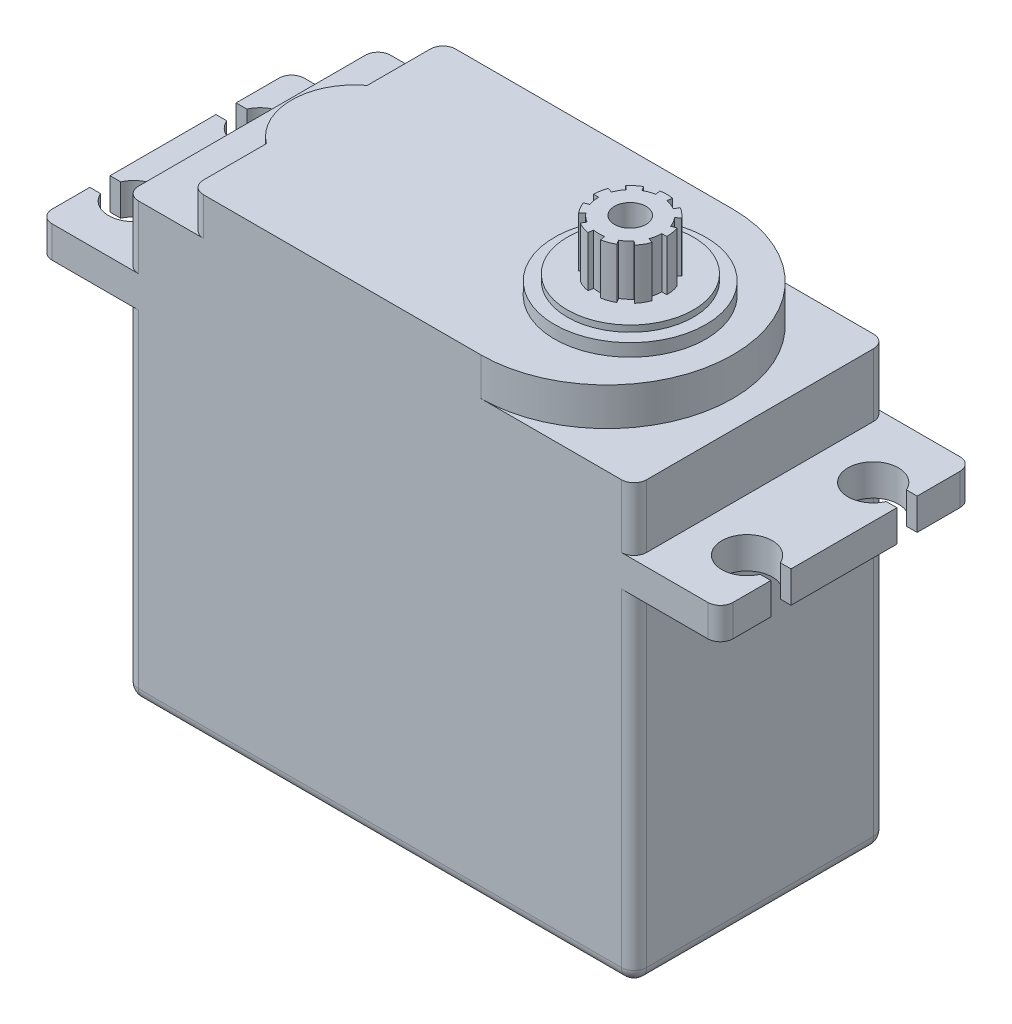
from build123d import *

# Parameters (mm, degrees)
EXTRUDE_1_DEPTH        = 20
FILLET_1_R             = 1
CUT_EXTRUDE_1_DEPTH    = 20
SKETCH_3_W             = 51.867663345
SKETCH_3_H             = 35.261757523
CUT_EXTRUDE_2_DEPTH    = 3
SKETCH_4_R             = 6
EXTRUDE_2_DEPTH        = 1
SKETCH_5_R             = 5
EXTRUDE_3_DEPTH        = 0.5
SKETCH_6_R             = 1
EXTRUDE_4_DEPTH        = 4
HOLE_WIZARD_M3_1_D     = 2.5
HOLE_WIZARD_M3_1_DEPTH = 7.5
HOLE_WIZARD_M3_1_TIP   = 0.751075774


with BuildPart() as part:
    # 草图1 → 凸台-拉伸1 (new body)
    with BuildSketch(Plane.XY):
        Polygon((20.15, 8), (27, 8), (27, 10.5), (20.15, 10.5), (20.15, 18.5), (-20.15, 18.5), (-20.15, 10.5), (-27, 10.5), (-27, 8), (-20.15, 8), (-20.15, -19), (20.15, -19), align=None)
    extrude(amount=EXTRUDE_1_DEPTH)

    # 圆角1
    fillet_1_edges = [part.edges().sort_by_distance(p)[0] for p in [
        (-27, 9.25, 20),
        (20.15, 14.5, 0),
        (27, 9.25, 0),
        (20.15, -5.5, 0),
        (0, -19, 0),
        (-20.15, -5.5, 0),
        (-27, 9.25, 0),
        (-20.15, 14.5, 0),
        (-20.15, -5.5, 20),
        (0, -19, 20),
        (-20.15, 18.5, 10),
        (20.15, 18.5, 10),
        (20.15, -19, 10),
        (-20.15, -19, 10),
        (20.15, -5.5, 20),
        (27, 9.25, 20),
        (20.15, 14.5, 20),
        (-20.15, 14.5, 20),
    ]]
    fillet(fillet_1_edges, radius=FILLET_1_R)

    # 草图2 → 切除-拉伸1 (cut)
    with BuildSketch(Plane(origin=(0, 10.5, 0), x_dir=(1, 0, 0), z_dir=(0, 1, 0))):
        with BuildLine():
            Line((-26.148030278, -4.4), (-29.222738853, -4.4))
            Line((-29.222738853, -4.4), (-29.222738853, -6))
            Line((-29.222738853, -6), (-26.148030278, -6))
            ThreePointArc((-26.148030278, -6), (-22.315, -5.2), (-26.148030278, -4.4))
        make_face()
        with BuildLine():
            Line((-26.148030278, -14.4), (-29.222738853, -14.4))
            Line((-29.222738853, -14.4), (-29.222738853, -16))
            Line((-29.222738853, -16), (-26.148030278, -16))
            ThreePointArc((-26.148030278, -16), (-22.315, -15.2), (-26.148030278, -14.4))
        make_face()
        with BuildLine():
            Line((26.148030278, -16), (29.222738853, -16))
            Line((29.222738853, -16), (29.222738853, -14.4))
            Line((29.222738853, -14.4), (26.148030278, -14.4))
            ThreePointArc((26.148030278, -14.4), (22.315, -15.2), (26.148030278, -16))
        make_face()
        with BuildLine():
            Line((29.222738853, -4.4), (29.222738853, -6))
            Line((29.222738853, -6), (26.148030278, -6))
            ThreePointArc((26.148030278, -6), (22.315, -5.2), (26.148030278, -4.4))
            Line((26.148030278, -4.4), (29.222738853, -4.4))
        make_face()
    extrude(amount=-CUT_EXTRUDE_1_DEPTH, mode=Mode.SUBTRACT)

    # 草图3 → 切除-拉伸2 (cut)
    with BuildSketch(Plane(origin=(0, 18.5, 0), x_dir=(1, 0, 0), z_dir=(0, 1, 0))):
        with Locations((-0.933831673, -10.85793672)):
            Rectangle(SKETCH_3_W, SKETCH_3_H)
        with BuildLine():
            Line((-14, 0), (8, 0))
            ThreePointArc((8, 0), (18, -10), (8, -20))
            Line((8, -20), (-14, -20))
            ThreePointArc((-14, -20), (-14.707106781, -19.707106781), (-15, -19))
            Line((-15, -19), (-15, -14))
            ThreePointArc((-15, -14), (-17, -10), (-15, -6))
            Line((-15, -6), (-15, -1))
            ThreePointArc((-15, -1), (-14.707106781, -0.292893219), (-14, 0))
        make_face(mode=Mode.SUBTRACT)
    extrude(amount=-CUT_EXTRUDE_2_DEPTH, mode=Mode.SUBTRACT)

    # 草图4 → 凸台-拉伸2 (add)
    with BuildSketch(Plane(origin=(0, 18.5, 0), x_dir=(1, 0, 0), z_dir=(0, 1, 0))):
        with Locations((9.85, -10)):
            Circle(SKETCH_4_R)
    extrude(amount=EXTRUDE_2_DEPTH)

    # 草图5 → 凸台-拉伸3 (add)
    with BuildSketch(Plane(origin=(0, 19.5, 0), x_dir=(1, 0, 0), z_dir=(0, 1, 0))):
        with Locations(Location((9.851314919, -9.987632383, 0), (0, 0, 270))):
            Circle(SKETCH_5_R)
    extrude(amount=EXTRUDE_3_DEPTH)

    # 草图6 → 凸台-拉伸4 (add)
    with BuildSketch(Plane(origin=(0, 20, 0), x_dir=(1, 0, 0), z_dir=(0, 1, 0))):
        with BuildLine():
            Line((10.284120444, -7.537980617), (10.353579715, -7.144057516))
            ThreePointArc((10.353579715, -7.144057516), (9.85, -7.1), (9.346420285, -7.144057516))
            Line((9.346420285, -7.144057516), (9.415879556, -7.537980617))
            ThreePointArc((9.415879556, -7.537980617), (8.994949642, -7.650768448), (8.6, -7.834936491))
            Line((8.6, -7.834936491), (8.4, -7.488526329))
            ThreePointArc((8.4, -7.488526329), (7.985915932, -7.778471115), (7.628471115, -8.135915932))
            Line((7.628471115, -8.135915932), (7.934888892, -8.393030976))
            ThreePointArc((7.934888892, -8.393030976), (7.684936491, -8.75), (7.500768448, -9.144949642))
            Line((7.500768448, -9.144949642), (7.1248914, -9.008141584))
            ThreePointArc((7.1248914, -9.008141584), (6.994057516, -9.496420285), (6.95, -10))
            Line((6.95, -10), (7.35, -10))
            ThreePointArc((7.35, -10), (7.387980617, -10.434120444), (7.500768448, -10.855050358))
            Line((7.500768448, -10.855050358), (7.1248914, -10.991858416))
            ThreePointArc((7.1248914, -10.991858416), (7.338526329, -11.45), (7.628471115, -11.864084068))
            Line((7.628471115, -11.864084068), (7.934888892, -11.606969024))
            ThreePointArc((7.934888892, -11.606969024), (8.243030976, -11.915111108), (8.6, -12.165063509))
            Line((8.6, -12.165063509), (8.4, -12.511473671))
            ThreePointArc((8.4, -12.511473671), (8.858141584, -12.7251086), (9.346420285, -12.855942484))
            Line((9.346420285, -12.855942484), (9.415879556, -12.462019383))
            ThreePointArc((9.415879556, -12.462019383), (9.85, -12.5), (10.284120444, -12.462019383))
            Line((10.284120444, -12.462019383), (10.353579715, -12.855942484))
            ThreePointArc((10.353579715, -12.855942484), (10.841858416, -12.7251086), (11.3, -12.511473671))
            Line((11.3, -12.511473671), (11.1, -12.165063509))
            ThreePointArc((11.1, -12.165063509), (11.456969024, -11.915111108), (11.765111108, -11.606969024))
            Line((11.765111108, -11.606969024), (12.071528885, -11.864084068))
            ThreePointArc((12.071528885, -11.864084068), (12.361473671, -11.45), (12.5751086, -10.991858416))
            Line((12.5751086, -10.991858416), (12.199231552, -10.855050358))
            ThreePointArc((12.199231552, -10.855050358), (12.312019383, -10.434120444), (12.35, -10))
            Line((12.35, -10), (12.75, -10))
            ThreePointArc((12.75, -10), (12.705942484, -9.496420285), (12.5751086, -9.008141584))
            Line((12.5751086, -9.008141584), (12.199231552, -9.144949642))
            ThreePointArc((12.199231552, -9.144949642), (12.015063509, -8.75), (11.765111108, -8.393030976))
            Line((11.765111108, -8.393030976), (12.071528885, -8.135915932))
            ThreePointArc((12.071528885, -8.135915932), (11.714084068, -7.778471115), (11.3, -7.488526329))
            Line((11.3, -7.488526329), (11.1, -7.834936491))
            ThreePointArc((11.1, -7.834936491), (10.705050358, -7.650768448), (10.284120444, -7.537980617))
        make_face()
        with Locations(Location((9.85, -10, 0), (0, 0, 270))):
            Circle(SKETCH_6_R, mode=Mode.SUBTRACT)
    extrude(amount=EXTRUDE_4_DEPTH)

    # M3 螺纹孔1
    with Locations(Plane(origin=(9.85, 24, 10), x_dir=(0, 0, 1), z_dir=(0, 1, 0))):
        with Locations((0, 0)):
            Hole(HOLE_WIZARD_M3_1_D / 2, depth=HOLE_WIZARD_M3_1_DEPTH)
            with Locations((0, 0, -(HOLE_WIZARD_M3_1_DEPTH + HOLE_WIZARD_M3_1_TIP / 2))):  # 118° drill point
                Cone(0, HOLE_WIZARD_M3_1_D / 2, HOLE_WIZARD_M3_1_TIP, mode=Mode.SUBTRACT)


solid = part.part
